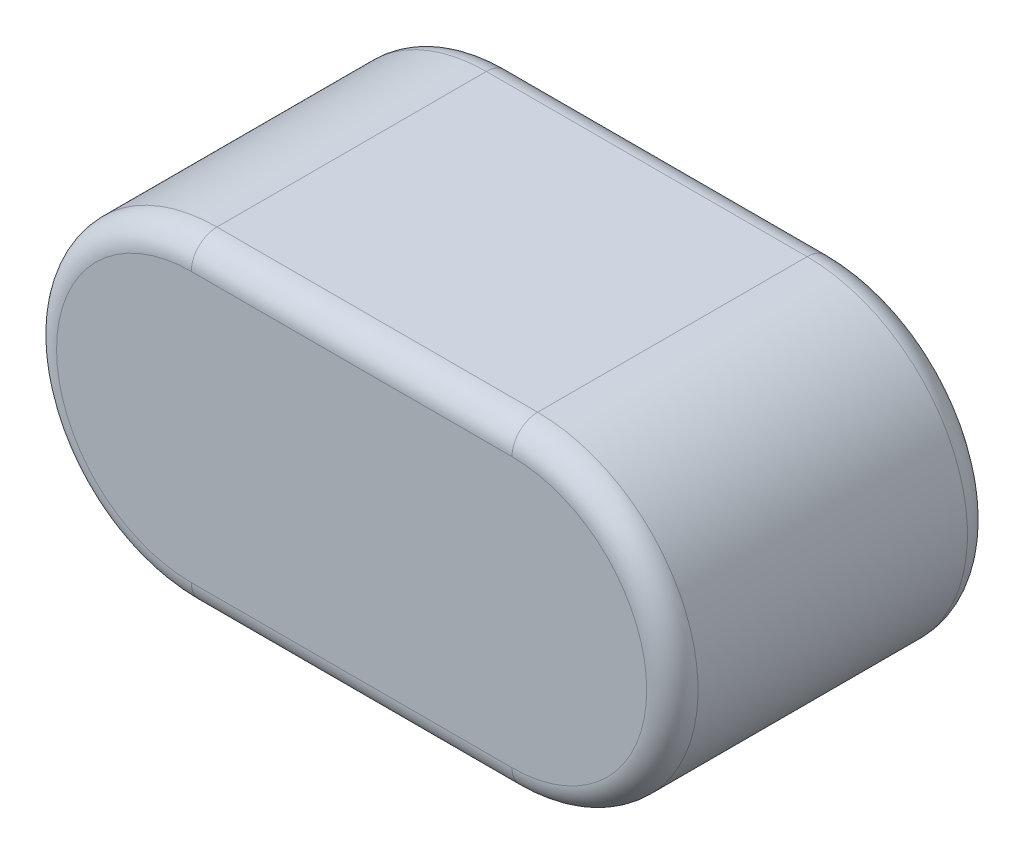
SolidWorks part; units mm, degrees
ref_plane "基准面1" through (0, 0, 0) normal (0, 0, 1) x (1, 0, 0)
ref_plane "基准面2" through (0, 0, 0) normal (0, 1, 0) x (1, 0, 0)
ref_plane "基准面3" through (0, 0, 0) normal (1, 0, 0) x (0, 0, -1)
sketch "尺寸草图" plane through (0, 0, 0) normal (0, 0, 1) x (1, 0, 0)
  line L0 (-5, 0) -> (5, 0) construction
  point P3 (-5, 0)
  point P4 (-0.4, 0)
  point P5 (0, 0)
  point P8 (-5, 0)
  point P11 (0, 0)
sketch "草图1" plane through (0, 0, 0) normal (0, 0, 1) x (1, 0, 0)
  line L0 (-28.0599, 0) -> (30.562, 0) construction
  line L1 (-2.5, 2.5) -> (2.5, 2.5)
  line L2 (-2.5, -2.5) -> (2.5, -2.5)
  line L3 (0, 2.9108) -> (0, -2.1805) construction
  arc A0 (-2.5, 2.5) -> (-2.5, -2.5) centre (-2.5, 0) ccw
  arc A1 (2.5, 2.5) -> (2.5, -2.5) centre (2.5, 0) cw
extrude "基体-拉伸" add sketch "草图1" along normal blind 5
fillet "圆角1" radius 0.4 8 edges at (5, 0, 5) (0, 2.5, 5) (-5, 0, 5) (0, 2.5, 0) (5, 0, 0) (0, -2.5, 0) (-5, 0, 0) (0, -2.5, 5)
equation "\"D3@草图1\" = \"L@尺寸草图\""
equation "\"D1@草图1\" = \"b@尺寸草图\" / 2"
equation "\"D1@圆角1\" = \"r@尺寸草图\""
equation "\"D1@基体-拉伸\" = \"h@尺寸草图\""
